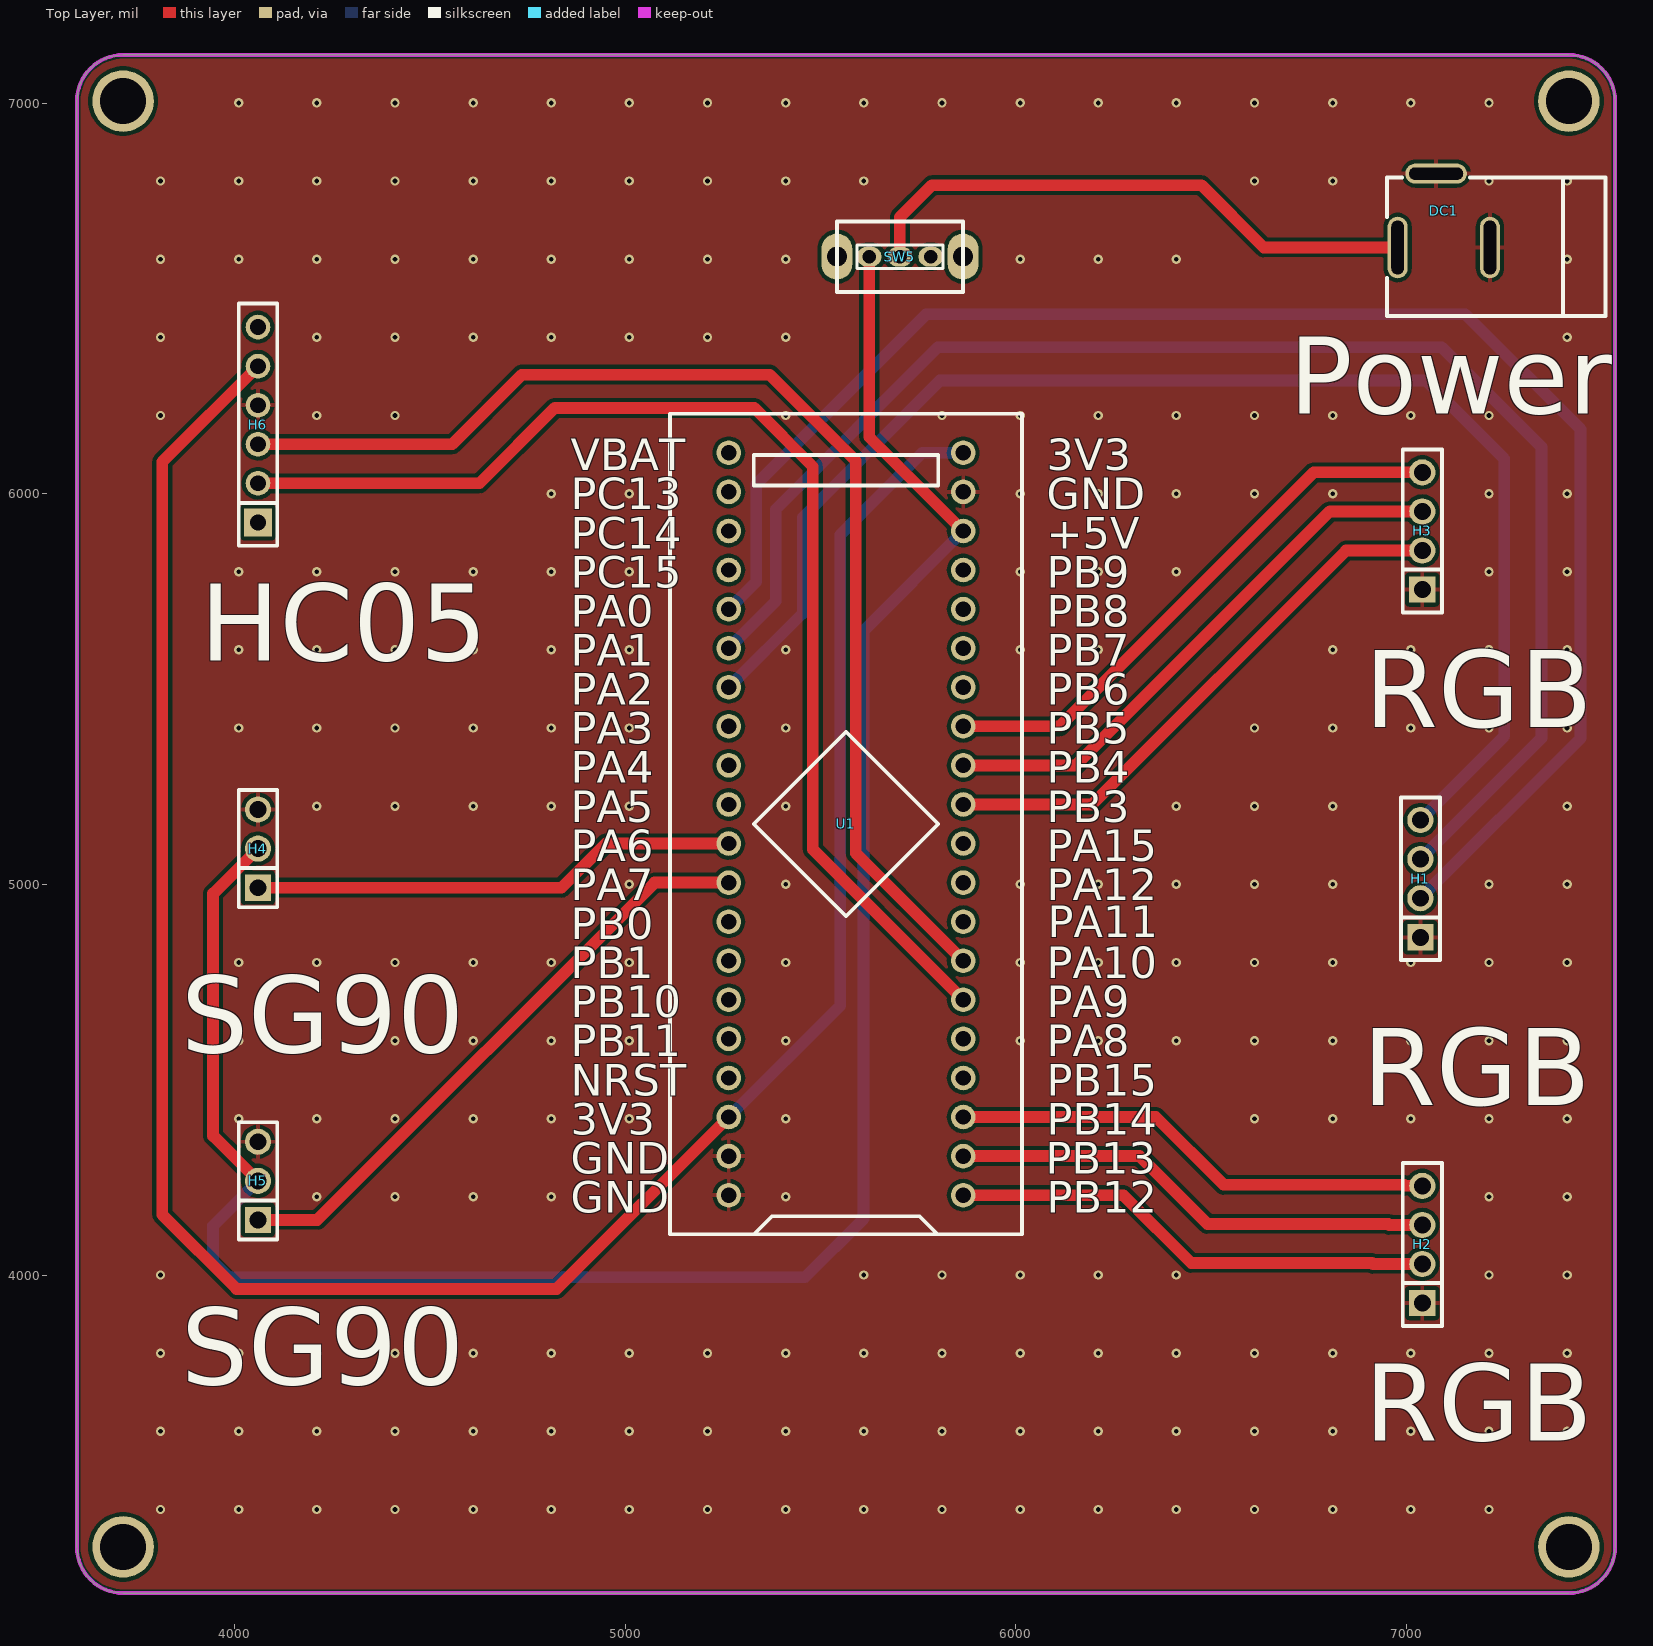
[diagram p0: Top Layer view]
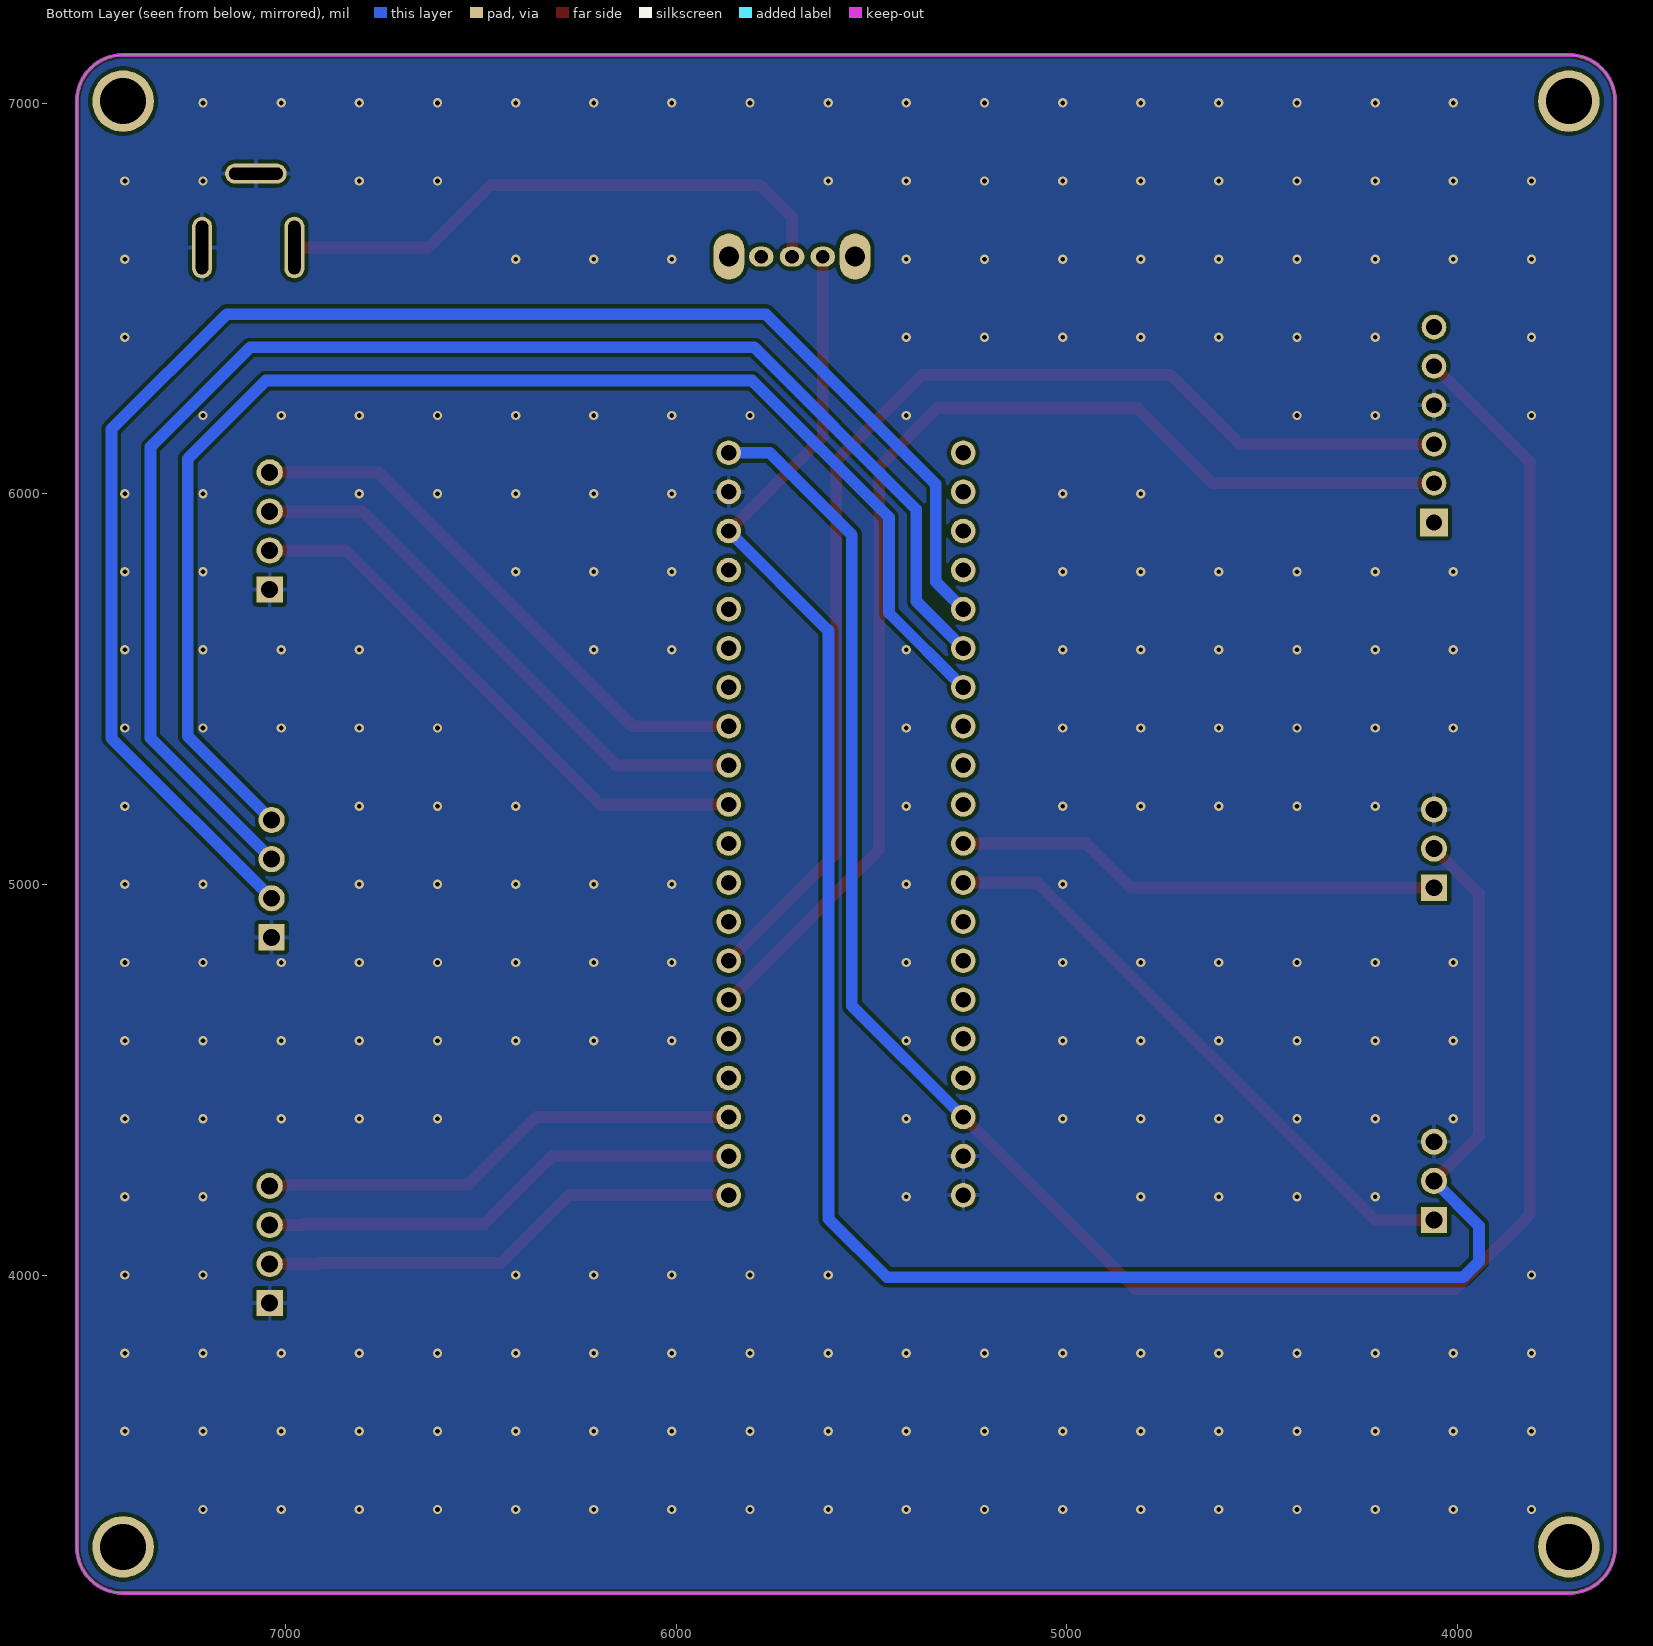
[diagram p1: Bottom Layer view, seen from below]
# Altium PCB MISC51537.pcbdoc
Units mil, origin at the board's own origin, x right, y up, seen from the top; angles counter-clockwise.
Board outline 3937.01 x 3937.01 mil, 2 copper layers (Top Layer, Bottom Layer), stack 62.206 mil thick; 9 components, 38 nets, 76 pads, 242 vias.

## Layer stack, top to bottom
Top Solder Mask Layer: solder mask 0.394, Dk 3.3
Top Layer: signal copper 1.379
Dielectric1: surface 59.449, FR4, Dk 4.5
Bottom Layer: signal copper 1.378
Bottom Solder Mask Layer: solder mask 0.394, Dk 3.3

## Board outline
3714.61,7123.5 ccw(c3714.61,7005.39) 3596.5,7005.39 3596.5,3304.61 ccw(c3714.61,3304.61) 3714.61,3186.5 7415.39,3186.5 ccw(c7415.39,3304.61) 7533.5,3304.61 7533.5,7005.39 ccw(c7415.39,7005.39) 7415.39,7123.5 3714.61,7123.5

## Design rules (kind name [scope] priority, off if disabled: settings)
BoardOutlineClearance copperThickness2oz_1 [All] p2 off: genericclearance=7.99 ignorepadtopadclearanceinfootprint=FALSE except(0: Arc-SplitContinuation Track-SplitContinuation SMDPad-SplitContinuation THPad-SplitContinuation Via-SplitContinuation Fill-SplitContinuation Region-SplitContinuation Poly-SplitContinuation Text-SplitContinuation Hole-SplitContinuation; 5.98: Arc-CutoutEdge Track-CutoutEdge SMDPad-CutoutEdge THPad-CutoutEdge Via-CutoutEdge Text-CutoutEdge; 6.9: Hole-OutlineEdge Hole-CutoutEdge; 10: Poly-OutlineEdge Poly-CutoutEdge; 11.81: Arc-OutlineEdge Track-OutlineEdge SMDPad-OutlineEdge THPad-OutlineEdge Via-OutlineEdge Fill-OutlineEdge Region-OutlineEdge Text-OutlineEdge Fill-CutoutEdge Region-CutoutEdge)
BoardOutlineClearance Plane_innerPlane_1 [All] p4 off: genericclearance=4.02 ignorepadtopadclearanceinfootprint=FALSE except(0: Arc-SplitContinuation Track-SplitContinuation SMDPad-SplitContinuation THPad-SplitContinuation Via-SplitContinuation Fill-SplitContinuation Region-SplitContinuation Poly-SplitContinuation Text-SplitContinuation Hole-SplitContinuation; 5.98: Arc-CutoutEdge Track-CutoutEdge SMDPad-CutoutEdge THPad-CutoutEdge Via-CutoutEdge Text-CutoutEdge; 6.9: Hole-OutlineEdge Hole-CutoutEdge; 10: Poly-OutlineEdge Poly-CutoutEdge; 11.81: Arc-OutlineEdge Track-OutlineEdge SMDPad-OutlineEdge THPad-OutlineEdge Via-OutlineEdge Fill-OutlineEdge Region-OutlineEdge Text-OutlineEdge Fill-CutoutEdge Region-CutoutEdge)
BoardOutlineClearance Copper_copperRegion_1 [All] p6 off: genericclearance=4.02 ignorepadtopadclearanceinfootprint=FALSE except(0: Arc-SplitContinuation Track-SplitContinuation SMDPad-SplitContinuation THPad-SplitContinuation Via-SplitContinuation Fill-SplitContinuation Region-SplitContinuation Poly-SplitContinuation Text-SplitContinuation Hole-SplitContinuation; 5.98: Arc-CutoutEdge Track-CutoutEdge SMDPad-CutoutEdge THPad-CutoutEdge Via-CutoutEdge Text-CutoutEdge; 6.9: Hole-OutlineEdge Hole-CutoutEdge; 10: Poly-OutlineEdge Poly-CutoutEdge; 11.81: Arc-OutlineEdge Track-OutlineEdge SMDPad-OutlineEdge THPad-OutlineEdge Via-OutlineEdge Fill-OutlineEdge Region-OutlineEdge Text-OutlineEdge Fill-CutoutEdge Region-CutoutEdge)
BoardOutlineClearance copperThickness1oz_1 [All] p8: genericclearance=4.02 ignorepadtopadclearanceinfootprint=FALSE except(0: Arc-SplitContinuation Track-SplitContinuation SMDPad-SplitContinuation THPad-SplitContinuation Via-SplitContinuation Fill-SplitContinuation Region-SplitContinuation Poly-SplitContinuation Text-SplitContinuation Hole-SplitContinuation; 5.98: Arc-CutoutEdge Track-CutoutEdge SMDPad-CutoutEdge THPad-CutoutEdge Via-CutoutEdge Text-CutoutEdge; 6.9: Hole-OutlineEdge Hole-CutoutEdge; 10: Poly-OutlineEdge Poly-CutoutEdge; 11.81: Arc-OutlineEdge Track-OutlineEdge SMDPad-OutlineEdge THPad-OutlineEdge Via-OutlineEdge Fill-OutlineEdge Region-OutlineEdge Text-OutlineEdge Fill-CutoutEdge Region-CutoutEdge)
Clearance copperThickness2oz [All] p1 off: gap=7.99 ignorepadtopadclearanceinfootprint=FALSE except(5.98: SMDPad-Track SMDPad-SMDPad THPad-Track SMDPad-THPad THPad-THPad Track-Via SMDPad-Via THPad-Via Via-Via Fill-SMDPad Region-SMDPad Fill-THPad Region-THPad Fill-Via Region-Via Fill-Fill Fill-Region Region-Region Arc-Track Arc-SMDPad Arc-THPad Arc-Via Fill-Arc Region-Arc Arc-Arc Text-Track SMDPad-Text Text-THPad Text-Via Fill-Text Region-Text Arc-Text Text-Text; 6.9: Hole-Track Hole-SMDPad Hole-THPad Hole-Via Fill-Hole Region-Hole Hole-Arc Hole-Text; 10: Poly-Track Poly-SMDPad Poly-THPad Poly-Via Poly-Fill Poly-Region Poly-Poly Poly-Arc Poly-Text Poly-Hole; 11.81: Fill-Track Region-Track)
Clearance Plane_innerPlane [All] p3 off: gap=4.02 ignorepadtopadclearanceinfootprint=FALSE except(5.98: SMDPad-Track SMDPad-SMDPad THPad-Track SMDPad-THPad THPad-THPad Track-Via SMDPad-Via THPad-Via Via-Via Fill-SMDPad Region-SMDPad Fill-THPad Region-THPad Fill-Via Region-Via Fill-Fill Fill-Region Region-Region Arc-Track Arc-SMDPad Arc-THPad Arc-Via Fill-Arc Region-Arc Arc-Arc Text-Track SMDPad-Text Text-THPad Text-Via Fill-Text Region-Text Arc-Text Text-Text; 6.9: Hole-Track Hole-SMDPad Hole-THPad Hole-Via Fill-Hole Region-Hole Hole-Arc Hole-Text; 10: Poly-Track Poly-SMDPad Poly-THPad Poly-Via Poly-Fill Poly-Region Poly-Poly Poly-Arc Poly-Text Poly-Hole; 11.81: Fill-Track Region-Track)
Clearance Copper_copperRegion [All] p5 off: gap=4.02 ignorepadtopadclearanceinfootprint=FALSE except(5.98: SMDPad-Track SMDPad-SMDPad THPad-Track SMDPad-THPad THPad-THPad Track-Via SMDPad-Via THPad-Via Via-Via Fill-SMDPad Region-SMDPad Fill-THPad Region-THPad Fill-Via Region-Via Fill-Fill Fill-Region Region-Region Arc-Track Arc-SMDPad Arc-THPad Arc-Via Fill-Arc Region-Arc Arc-Arc Text-Track SMDPad-Text Text-THPad Text-Via Fill-Text Region-Text Arc-Text Text-Text; 6.9: Hole-Track Hole-SMDPad Hole-THPad Hole-Via Fill-Hole Region-Hole Hole-Arc Hole-Text; 10: Poly-Track Poly-SMDPad Poly-THPad Poly-Via Poly-Fill Poly-Region Poly-Poly Poly-Arc Poly-Text Poly-Hole; 11.81: Fill-Track Region-Track)
Clearance copperThickness1oz [All] p7: gap=4.02 ignorepadtopadclearanceinfootprint=FALSE except(5.98: SMDPad-Track SMDPad-SMDPad THPad-Track SMDPad-THPad THPad-THPad Track-Via SMDPad-Via THPad-Via Via-Via Fill-SMDPad Region-SMDPad Fill-THPad Region-THPad Fill-Via Region-Via Fill-Fill Fill-Region Region-Region Arc-Track Arc-SMDPad Arc-THPad Arc-Via Fill-Arc Region-Arc Arc-Arc Text-Track SMDPad-Text Text-THPad Text-Via Fill-Text Region-Text Arc-Text Text-Text; 6.9: Hole-Track Hole-SMDPad Hole-THPad Hole-Via Fill-Hole Region-Hole Hole-Arc Hole-Text; 10: Poly-Track Poly-SMDPad Poly-THPad Poly-Via Poly-Fill Poly-Region Poly-Poly Poly-Arc Poly-Text Poly-Hole; 11.81: Fill-Track Region-Track)
DiffPairsRouting differentialPair [All] p1: maxlimit=6 minlimit=6 mostfreqgap=6 toplayer_minwidth=5 toplayer_prefwidth=10 toplayer_maxwidth=100 toplayer_mingap=6 toplayer_prefgap=6 toplayer_maxgap=6 bottomlayer_minwidth=5 bottomlayer_prefwidth=10 bottomlayer_maxwidth=100 bottomlayer_mingap=6 bottomlayer_prefgap=6 bottomlayer_maxgap=6 maxuncoupledlength=10
HoleToHoleClearance otherClearance [All] p1: gap=11.81 allowstackedmicrovias=TRUE
Length netLength [All] p1: minlimit=0 maxlimit=0
PasteMaskExpansion pasteMaskExpansion [All] p1: expansion=0
PlaneConnect innerPlane [All] p1: planeconnectstyle=Relief reliefexpansion=20 reliefentries=4 reliefconductorwidth=10 reliefairgap=10
PolygonConnect copperRegion [All] p1: connectstyle=Relief reliefconductorwidth=10 reliefentries=4 polygonreliefangle="90 Angle" airgapwidth=10 via.connectstyle=Relief via.reliefconductorwidth=10 via.reliefentries=4 via.polygonreliefangle="90 Angle" via.airgapwidth=10
RoutingVias viaSize [All] p1: holewidth=12.01 width=24.02 viastyle="Through Hole" minholewidth=11.81 minwidth=19.68 maxholewidth=248.03 maxwidth=393.7
SolderMaskExpansion solderMaskExpansion [IsVia] p1: expansion=-1000 istentingtop=TRUE
SolderMaskExpansion solderMaskExpansion [All] p2: expansion=2 istentingtop=FALSE
Width copperThickness2oz_2 [All] p1 off: maxlimit=100 minlimit=8 preferedwidth=10
Width copperThickness1oz_2 [All] p2: maxlimit=100 minlimit=5 preferedwidth=10

## Components (designator, comment, footprint, x,y, rotation, side; value= is the part's Value field where it differs from the comment)
DC1 "" DC-2.0 7100,6620 r0 top
H1 "" HDR-TH_4P-P2.54-V-F 7035,5015 r90 top
H2 "" HDR-TH_4P-P2.54-V-F 7040,4078.82 r90 top
H3 "" HDR-TH_4P-P2.54-V-F 7040,5905 r90 top
H4 "" HDR-TH_3P-P2.54-V-M 4060,5091.87 r90 top
H5 "" HDR-TH_3P-P2.54-V-M 4060,4241.71 r90 top
H6 "" HDR-TH_6P-P2.54-V-F 4060,6176.91 r90 top
SW5 "" 拨动开关 5697.9,6607.05 r0 top
U1 "STM32F103C8T6-Card" CONN-TH_L53.3-W22.9_STM32F103C8T6-CARD 5565,5155 r90 top

## Footprints (in the part's own frame and the unit in brackets; to place one, negate y for a bottom-side part, rotate by r counter-clockwise, add the part's x,y. Pads: shape width x height; smd on the part's side, far side on the other; paste and mask are expansions set on the pad)
CONN-TH_L53.3-W22.9_STM32F103C8T6-CARD [mm]
  round 1.6 hole 1: 1(-24.13,-7.62) 2(-21.59,-7.62) 3(-19.05,-7.62) 4(-16.51,-7.62) 5(-13.97,-7.62) 6(-11.43,-7.62) 7(-8.89,-7.62) 8(-6.35,-7.62) 9(-3.81,-7.62) 10(-1.27,-7.62) 11(1.27,-7.62) 12(3.81,-7.62) 13(6.35,-7.62) 14(8.89,-7.62) 15(11.43,-7.62) 16(13.97,-7.62) 17(16.51,-7.62) 18(19.05,-7.62) 19(21.59,-7.62) 20(24.13,-7.62) 21(24.13,7.62) 22(21.59,7.62) 23(19.05,7.62) 24(16.51,7.62) 25(13.97,7.62) 26(11.43,7.62) 27(8.89,7.62) 28(6.35,7.62) 29(3.81,7.62) 30(1.27,7.62) 31(-1.27,7.62) 32(-3.81,7.62) 33(-6.35,7.62) 34(-8.89,7.62) 35(-11.43,7.62) 36(-13.97,7.62) 37(-16.51,7.62) 38(-19.05,7.62) 39(-21.59,7.62) 40(-24.13,7.62)
  silkscreen extent -26.67,-11.43 26.67,11.43
DC-2.0 [mil]
  oval 157.5x51.2 hole 31.5 slot 137.8 at 0 deg paste+0 mask+2: 2(-24.7,199.5)
  oval 51.2x157.5 hole 31.5 slot 137.8 at 90 deg paste+0 mask+2: 3(113.1,10.5) 4(-123.1,10.5)
  silkscreen extent -151,-165 408,190
HDR-TH_3P-P2.54-V-M [mm]
  rect 1.7x1.7 hole 1.1: 1(-2.54,0)
  round 1.7 hole 1.1: 2(0,0) 3(2.54,0)
  silkscreen extent -3.81,-1.25 3.81,1.25
HDR-TH_4P-P2.54-V-F [mm]
  rect 1.7x1.7 hole 1.1: 1(-3.81,0)
  round 1.7 hole 1.1: 2(-1.27,0) 3(1.27,0) 4(3.81,0)
  silkscreen extent -5.29,-1.27 5.29,1.27
HDR-TH_6P-P2.54-V-F [mm]
  rect 1.8x1.8 hole 1.02: 1(-6.35,0)
  round 1.6 hole 1.02: 2(-3.81,0) 3(-1.27,0) 4(1.27,0) 5(3.81,0) 6(6.35,0)
  silkscreen extent -7.87,-1.25 7.87,1.25
拨动开关 [mil]
  oval 63x51.2 hole 35.4 paste+0 mask+2: 1(-73.4,0) 2(5,0) 3(84,0)
  oval 78.7x118.1 hole 51.2 paste+0 mask+2: 4(166.7,0) 5(-156.1,0)
  silkscreen extent -156,-90 167,90

## Free pads (board coordinates)
  round 157.48 hole 118.11: 1(3714.61,7005.39) 1(3714.61,3304.61) 1(7415.39,7005.39) 1(7415.39,3304.61)

## Via types
v1: diameter 24.02, hole 12, Top Layer to Bottom Layer, 242 vias

## Nets (pads, with @x,y where several pads share a name; then routed paths per layer and width w, separated by ;. In a path a pad name is that pad's centre, name@x,y a point inside that pad or via, vN(x,y) a via of type N, cw(c..) or ccw(c..) an arc to the next point about the centre after c; other vN are vias at no path point)
$1N17142: DC1.4 SW5.2 | length 1474.9
  Top Layer w30: SW5.2 5702.9,6707.9 5785,6790 6475,6790 6634.5,6630.5 DC1.4
+5V: H4.2 H5.2 SW5.1 U1.18 | length 5610.8
  Top Layer w30: H5.2 3945,4356.71 3945,4976.87 H4.2 ; SW5.1 5624.5,6145.5 U1.18
  Bottom Layer w30: H5.2 3945,4126.72 3945,4035 3985,3995 5460,3995 5610,4145 5610,5650 U1.18
GND: DC1.2 DC1.3 H1.1 H2.1 H3.1 H4.3 H5.3 H6.4 U1.19 U1.39 U1.40
  other v1: 3810.6,3400.6 4010.6,3400.6 4210.6,3400.6 4410.6,3400.6 4610.6,3400.6 4810.6,3400.6 5010.6,3400.6 5210.6,3400.6 5410.6,3400.6 5610.6,3400.6 5810.6,3400.6 6010.6,3400.6 6210.6,3400.6 6410.6,3400.6 6610.6,3400.6 6810.6,3400.6 7010.6,3400.6 7210.6,3400.6 3810.6,3600.6 4010.6,3600.6 4210.6,3600.6 4410.6,3600.6 4610.6,3600.6 4810.6,3600.6 5010.6,3600.6 5210.6,3600.6 5410.6,3600.6 5610.6,3600.6 5810.6,3600.6 6010.6,3600.6 6210.6,3600.6 6410.6,3600.6 6610.6,3600.6 6810.6,3600.6 7010.6,3600.6 7210.6,3600.6 7410.6,3600.6 3810.6,3800.6 4010.6,3800.6 4210.6,3800.6 4410.6,3800.6 4610.6,3800.6 4810.6,3800.6 5010.6,3800.6 5210.6,3800.6 5410.6,3800.6 5610.6,3800.6 5810.6,3800.6 6010.6,3800.6 6210.6,3800.6 6410.6,3800.6 6610.6,3800.6 6810.6,3800.6 7010.6,3800.6 7210.6,3800.6 7410.6,3800.6 3810.6,4000.6 5610.6,4000.6 5810.6,4000.6 6010.6,4000.6 6210.6,4000.6 6410.6,4000.6 7210.6,4000.6 7410.6,4000.6 4210.6,4200.6 4410.6,4200.6 4610.6,4200.6 4810.6,4200.6 5410.6,4200.6 7210.6,4200.6 7410.6,4200.6 4010.6,4400.6 4210.6,4400.6 4410.6,4400.6 4610.6,4400.6 4810.6,4400.6 5010.6,4400.6 5410.6,4400.6 6610.6,4400.6 6810.6,4400.6 7010.6,4400.6 7210.6,4400.6 7410.6,4400.6 4010.6,4600.6 4210.6,4600.6 4410.6,4600.6 4610.6,4600.6 4810.6,4600.6 5010.6,4600.6 5410.6,4600.6 6010.6,4600.6 6210.6,4600.6 6410.6,4600.6 6610.6,4600.6 6810.6,4600.6 7010.6,4600.6 7210.6,4600.6 7410.6,4600.6 4010.6,4800.6 4210.6,4800.6 4410.6,4800.6 4610.6,4800.6 4810.6,4800.6 5010.6,4800.6 5410.6,4800.6 6010.6,4800.6 6210.6,4800.6 6410.6,4800.6 6610.6,4800.6 6810.6,4800.6 7010.6,4800.6 7210.6,4800.6 7410.6,4800.6 5010.6,5000.6 5410.6,5000.6 6010.6,5000.6 6210.6,5000.6 6410.6,5000.6 6610.6,5000.6 6810.6,5000.6 7210.6,5000.6 7410.6,5000.6 4210.6,5200.6 4410.6,5200.6 4610.6,5200.6 4810.6,5200.6 5010.6,5200.6 5410.6,5200.6 6410.6,5200.6 6610.6,5200.6 6810.6,5200.6 7410.6,5200.6 4010.6,5400.6 4210.6,5400.6 4410.6,5400.6 4610.6,5400.6 4810.6,5400.6 5010.6,5400.6 5410.6,5400.6 6610.6,5400.6 6810.6,5400.6 7010.6,5400.6 7210.6,5400.6 7410.6,5400.6 4010.6,5600.6 4210.6,5600.6 4410.6,5600.6 4610.6,5600.6 4810.6,5600.6 5010.6,5600.6 5410.6,5600.6 6010.6,5600.6 6210.6,5600.6 6810.6,5600.6 7010.6,5600.6 7210.6,5600.6 7410.6,5600.6 4010.6,5800.6 4210.6,5800.6 4410.6,5800.6 4610.6,5800.6 4810.6,5800.6 5010.6,5800.6 6010.6,5800.6 6210.6,5800.6 6410.6,5800.6 7210.6,5800.6 7410.6,5800.6 4810.6,6000.6 5010.6,6000.6 6010.6,6000.6 6210.6,6000.6 6410.6,6000.6 6610.6,6000.6 6810.6,6000.6 7210.6,6000.6 7410.6,6000.6 3810.6,6200.6 4210.6,6200.6 4410.6,6200.6 5410.6,6200.6 5810.6,6200.6 6010.6,6200.6 6210.6,6200.6 6410.6,6200.6 6610.6,6200.6 6810.6,6200.6 7010.6,6200.6 7210.6,6200.6 3810.6,6400.6 4210.6,6400.6 4410.6,6400.6 4610.6,6400.6 4810.6,6400.6 5010.6,6400.6 5210.6,6400.6 5410.6,6400.6 7410.6,6400.6 3810.6,6600.6 4010.6,6600.6 4210.6,6600.6 4410.6,6600.6 4610.6,6600.6 4810.6,6600.6 5010.6,6600.6 5210.6,6600.6 5410.6,6600.6 6010.6,6600.6 6210.6,6600.6 6410.6,6600.6 7410.6,6600.6 3810.6,6800.6 4010.6,6800.6 4210.6,6800.6 4410.6,6800.6 4610.6,6800.6 4810.6,6800.6 5010.6,6800.6 5210.6,6800.6 5410.6,6800.6 5610.6,6800.6 6610.6,6800.6 6810.6,6800.6 7210.6,6800.6 7410.6,6800.6 4010.6,7000.6 4210.6,7000.6 4410.6,7000.6 4610.6,7000.6 4810.6,7000.6 5010.6,7000.6 5210.6,7000.6 5410.6,7000.6 5610.6,7000.6 5810.6,7000.6 6010.6,7000.6 6210.6,7000.6 6410.6,7000.6 6610.6,7000.6 6810.6,7000.6 7010.6,7000.6 7210.6,7000.6
NRST: U1.37
PA0: H1.2 U1.25 | length 4131.2
  Bottom Layer w30: U1.25 5335,5775 5335,6025 5770,6460 7150,6460 7445,6165 7445,5375 H1.2
PA1: H1.3 U1.26 | length 3825.6
  Bottom Layer w30: U1.26 5385,5725 5385,5960 5800,6375 7090,6375 7345,6120 7345,5375 H1.3
PA2: H1.4 U1.27 | length 3550.6
  Bottom Layer w30: U1.27 5455,5695 5455,5940 5805,6290 7050,6290 7250,6090 7250,5380 H1.4
PA3: U1.28
PA4: U1.29
PA5: U1.30
PA6: H4.1 U1.31 | length 1251.9
  Top Layer w30: H4.1 4836.87,4991.87 4950,5105 U1.31
PA7: H5.1 U1.32 | length 1562.6
  Top Layer w30: H5.1 4211.71,4141.71 5075,5005 U1.32
PA8: U1.5
PA9: H6.2 U1.6 | length 3086.6
  Top Layer w30: H6.2 4626.91,6026.91 4820,6220 5330,6220 5480,6070 5480,5090 U1.6
PA10: H6.3 U1.7 | length 3088.8
  Top Layer w30: H6.3 4556.91,6126.91 4735,6305 5370,6305 5590,6085 5590,5080 U1.7
PA11: U1.8
PA12: U1.9
PA15: U1.10
PB0: U1.33
PB1: U1.34
PB3: H3.2 U1.11 | length 1444.2
  Top Layer w30: U1.11 6195,5205 6845,5855 H3.2
PB4: H3.3 U1.12 | length 1444.2
  Top Layer w30: U1.12 6153.58,5305 6803.58,5955 H3.3
PB5: H3.4 U1.13 | length 1444.2
  Top Layer w30: U1.13 6112.16,5405 6762.16,6055 H3.4
PB6: U1.14
PB7: U1.15
PB8: U1.16
PB9: U1.17
PB10: U1.35
PB11: U1.36
PB12: H2.2 U1.1 | length 1248
  Top Layer w30: U1.1 6275,4205 6448.58,4031.42 6911.09,4031.42 6913.69,4028.82 H2.2
PB13: H2.3 U1.2 | length 1248
  Top Layer w30: U1.2 6316.42,4305 6490,4131.42 6952.51,4131.42 6955.11,4128.82 H2.3
PB14: H2.4 U1.3 | length 1248
  Top Layer w30: U1.3 6357.84,4405 6531.42,4231.42 6993.93,4231.42 6996.54,4228.82 H2.4
PB15: U1.4
PC13: U1.22
PC14: U1.23
PC15: U1.24
VBAT: U1.21
VCC: H6.5 U1.20 U1.38 | length 5994.4
  Top Layer w30: H6.5 3815,6081.91 3815,4155 4005,3965 4825,3965 U1.38
  Bottom Layer w30: U1.38 5550,4690 5550,5895 5760,6105 U1.20
pads on no net: H6.1 H6.6 SW5.3 SW5.4 SW5.5

## Polygon pours and split planes (outlines as drawn)
GND on Bottom Layer (solid, remove dead copper, pour order 2): 3525,7245 3525,3080 7700,3080 7700,7245
GND on Top Layer (solid, remove dead copper, pour order 2): 3000,7415 3000,3000 7930,3000 7930,7415

## Keep-outs
Board Outline Layer:
  the board outline again, w10

## Silkscreen, mask and mechanical layers (free items; w line width, h text height)
Top Silkscreen Layer:
  text "Power interface" at 6700,6205 h196.85
  text "VBAT" at 4860.95,6060 h80
  text "3V3" at 6079.16,6060 h80
  text "PC13" at 4860.95,5960 h80
  text "GND" at 6079.16,5960 h80
  text "PC14" at 4860.95,5860 h80
  text "+5V" at 6079.16,5860 h80
  text "PC15" at 4860.95,5760 h80
  text "PB9" at 6079.16,5760 h80
  text "PA0" at 4860.95,5660 h80
  text "PB8" at 6079.16,5660 h80
  text "HC05" at 3912.66,5573.09 h196.85
  text "PA1" at 4860.95,5560 h80
  text "PB7" at 6079.16,5560 h80
  text "PA2" at 4860.95,5460 h80
  text "PB6" at 6079.16,5460 h80
  text "RGB" at 6892.66,5402.76 h196.85
  text "PA3" at 4860.95,5360 h80
  text "PB5" at 6079.16,5360 h80
  text "PA4" at 4860.95,5260 h80
  text "PB4" at 6079.16,5260 h80
  text "PA5" at 4860.95,5160 h80
  text "PB3" at 6079.16,5160 h80
  text "PA6" at 4860.95,5060 h80
  text "PA15" at 6079.16,5060 h80
  text "PA7" at 4860.95,4960 h80
  text "PA12" at 6079.16,4960 h80
  text "PA11" at 6080.95,4865 h80
  text "PB0" at 4860.95,4860 h80
  text "PB1" at 4860.95,4760 h80
  text "PA10" at 6079.16,4760 h80
  text "PB10" at 4860.95,4660 h80
  text "PA9" at 6079.16,4660 h80
  text "SG90" at 3863.9,4570.16 h196.85
  text "PB11" at 4860.95,4560 h80
  text "PA8" at 6079.16,4560 h80
  text "NRST" at 4860.95,4460 h80
  text "PB15" at 6079.16,4460 h80
  text "RGB" at 6887.66,4435.32 h196.85
  text "3V3" at 4860.95,4360 h80
  text "PB14" at 6079.16,4360 h80
  text "GND" at 4860.95,4260 h80
  text "PB13" at 6075.95,4260 h80
  text "GND" at 4860.95,4160 h80
  text "PB12" at 6079.16,4160 h80
  text "SG90" at 3863.9,3720 h196.85
  text "RGB" at 6892.66,3576.57 h196.85